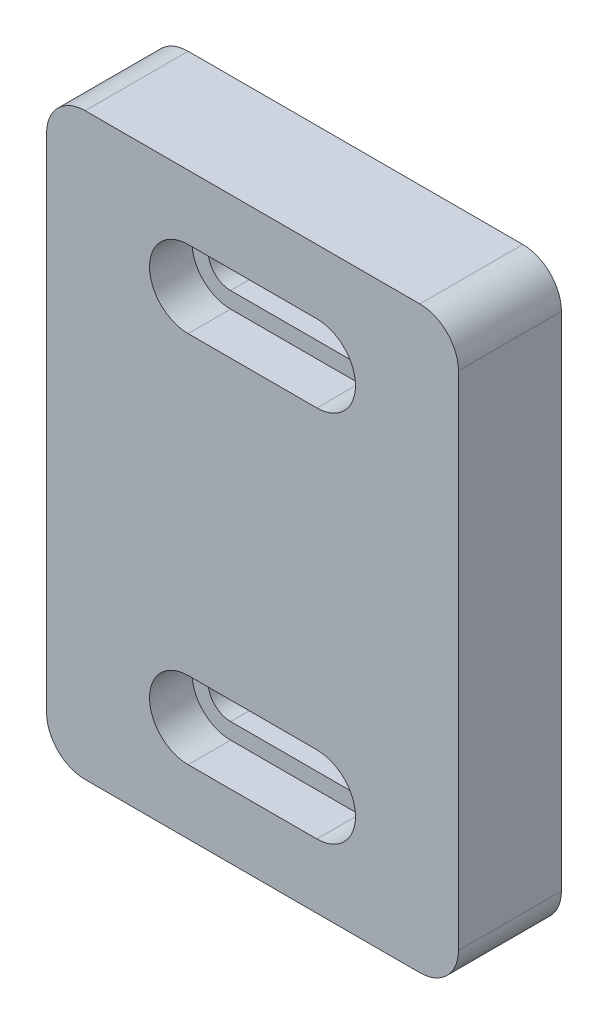
from build123d import *

# Parameters (mm, degrees)
SKETCH1_W           = 32
SKETCH1_H           = 45
BOSS_EXTRUDE1_DEPTH = 8
FILLET1_R           = 3
CUT_EXTRUDE1_DEPTH  = 29.744564704
CUT_EXTRUDE2_DEPTH  = 3.3


with BuildPart() as part:
    # Sketch1 → Boss-Extrude1 (new body)
    with BuildSketch(Plane.XY):
        Rectangle(SKETCH1_W, SKETCH1_H)
    extrude(amount=BOSS_EXTRUDE1_DEPTH)

    # Fillet1
    fillet1_edges = [part.edges().sort_by_distance(p)[0] for p in [
        (-16, 22.5, 4),
        (16, 22.5, 4),
        (16, -22.5, 4),
        (-16, -22.5, 4),
    ]]
    fillet(fillet1_edges, radius=FILLET1_R)

    # Sketch2 → Cut-Extrude1 (cut, through all)
    with BuildSketch(Plane.XY.offset(8)):
        with BuildLine():
            Line((-5, 16.25), (5, 16.25))
            ThreePointArc((5, 16.25), (6.75, 14.5), (5, 12.75))
            Line((5, 12.75), (-5, 12.75))
            ThreePointArc((-5, 12.75), (-6.75, 14.5), (-5, 16.25))
        make_face()
        with BuildLine():
            Line((-5, -12.75), (5, -12.75))
            ThreePointArc((5, -12.75), (6.75, -14.5), (5, -16.25))
            Line((5, -16.25), (-5, -16.25))
            ThreePointArc((-5, -16.25), (-6.75, -14.5), (-5, -12.75))
        make_face()
    extrude(amount=-CUT_EXTRUDE1_DEPTH, mode=Mode.SUBTRACT)

    # Sketch3 → Cut-Extrude2 (cut)
    with BuildSketch(Plane.XY.offset(8)):
        with BuildLine():
            Line((-5, 17.5), (5, 17.5))
            ThreePointArc((5, 17.5), (8, 14.5), (5, 11.5))
            Line((5, 11.5), (-5, 11.5))
            ThreePointArc((-5, 11.5), (-8, 14.5), (-5, 17.5))
        make_face()
        with BuildLine():
            Line((-5, -11.5), (5, -11.5))
            ThreePointArc((5, -11.5), (8, -14.5), (5, -17.5))
            Line((5, -17.5), (-5, -17.5))
            ThreePointArc((-5, -17.5), (-8, -14.5), (-5, -11.5))
        make_face()
    extrude(amount=-CUT_EXTRUDE2_DEPTH, mode=Mode.SUBTRACT)


solid = part.part
